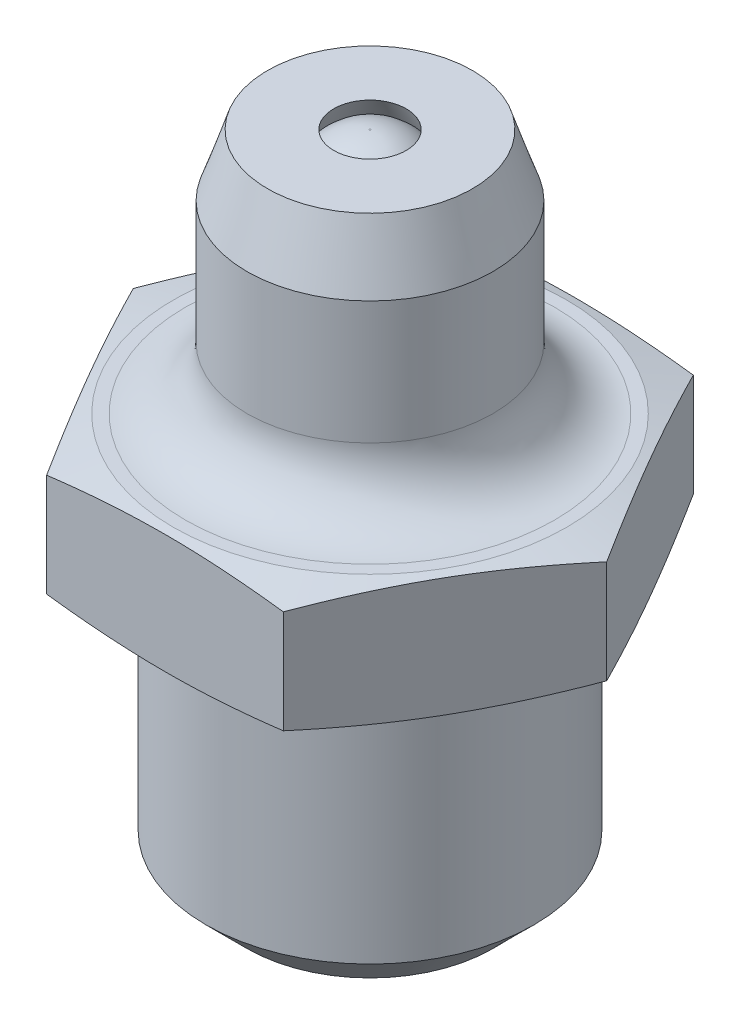
SolidWorks part; units mm, degrees
material "铜"
ref_plane "Front Plane" through (0, 0, 0) normal (0, 0, 1) x (1, 0, 0)
ref_plane "Top Plane" through (0, 0, 0) normal (0, 1, 0) x (1, 0, 0)
ref_plane "Right Plane" through (0, 0, 0) normal (1, 0, 0) x (0, 0, -1)
sketch "Sketch1" plane through (0, 0, 0) normal (0, 1, 0) x (1, 0, 0)
  circle A0 centre (0, 0) radius 4
  dimension "D1" = 8
extrude "Boss-Extrude1" add sketch "Sketch1" along normal blind 6.8
cosmetic thread "Cosmetic Thread1" parameters "D2"=6.647
sketch "Sketch2" plane through (0, 6.8, 0) normal (0, 1, 0) x (1, 0, 0)
  line L1 (2.8868, -5) -> (5.7735, 0)
  line L2 (5.7735, 0) -> (2.8868, 5)
  line L3 (2.8868, 5) -> (-2.8868, 5)
  line L4 (-2.8868, 5) -> (-5.7735, 0)
  line L5 (-5.7735, 0) -> (-2.8868, -5)
  line L6 (-2.8868, -5) -> (2.8868, -5)
  circle A0 centre (0, 0) radius 5 construction
  dimension "D1" = 10
extrude "Boss-Extrude2" add sketch "Sketch2" along normal blind 3
sketch "Sketch3" plane through (0, 0, 0) normal (0, 0, 1) x (1, 0, 0)
  line L0 (0, -1.8804) -> (0, 20.3927)
  line L3 (-2.8868, 9.8) -> (2.8868, 9.8) construction
  line L4 (0, 9.8) -> (0, 15.8)
  line L5 (0, 15.8) -> (2.5, 15.8)
  line L6 (2.5, 15.8) -> (3, 14.3)
  line L7 (3, 14.3) -> (3, 11.3)
  line L8 (0, 9.8) -> (5.0231, 9.8)
  line L9 (2.8868, 9.8) -> (5.7735, 9.8) construction
  line L10 (-4, 0) -> (4, 0) construction
  arc A0 (3, 11.3) -> (4.5003, 9.8) centre (4.5, 11.3) ccw
  dimension "D1" = 15.8
  dimension "D2" = 3
  dimension "D3" = 2.5
  dimension "D4" = 1.5
revolve "Revolve1" add sketch "Sketch3" angle 360 about L0
sketch "Sketch5" plane through (0, 0, 0) normal (1, 0, 0) x (0, 0, -1)
  line L0 (-4.8, 9.8) -> (-6.8, 9.3)
  line L1 (-6.8, 9.3) -> (-6.8, 9.8)
  line L2 (-6.8, 9.8) -> (-4.8, 9.8)
  line L3 (0, 16.9996) -> (0, -2.9721)
  line L4 (-4.8, 6.8) -> (-6.8, 6.8)
  line L5 (-6.8, 6.8) -> (-6.8, 7.3)
  line L6 (-6.8, 7.3) -> (-4.8, 6.8)
  line L7 (-5, 9.8) -> (0, 9.8) construction
  line L8 (-5, 6.8) -> (0, 6.8) construction
  dimension "D1" = 0.5
  dimension "D2" = 0.5
  dimension "D3" = 2
  dimension "D4" = 2
  dimension "D5" = 0.2
revolve "Cut-Revolve1" cut sketch "Sketch5" angle 360 about L3
chamfer "Chamfer1" distance 1 angle 45 1 edges at (0, 0, 4)
sketch "Sketch6" plane through (0, 0, 0) normal (1, 0, 0) x (0, 0, -1)
  line L0 (0, 16.9172) -> (0, -0.6474)
  line L1 (-1.293, 15.0184) -> (-0.8829, 15.8)
  line L2 (2.5, 15.8) -> (-2.5, 15.8) construction
  line L3 (-0.8829, 15.8) -> (-0.0201, 15.8)
  circle A0 centre (0, 14.34) radius 1.4602
revolve "Cut-Revolve4" cut sketch "Sketch6" angle 360 about L0
